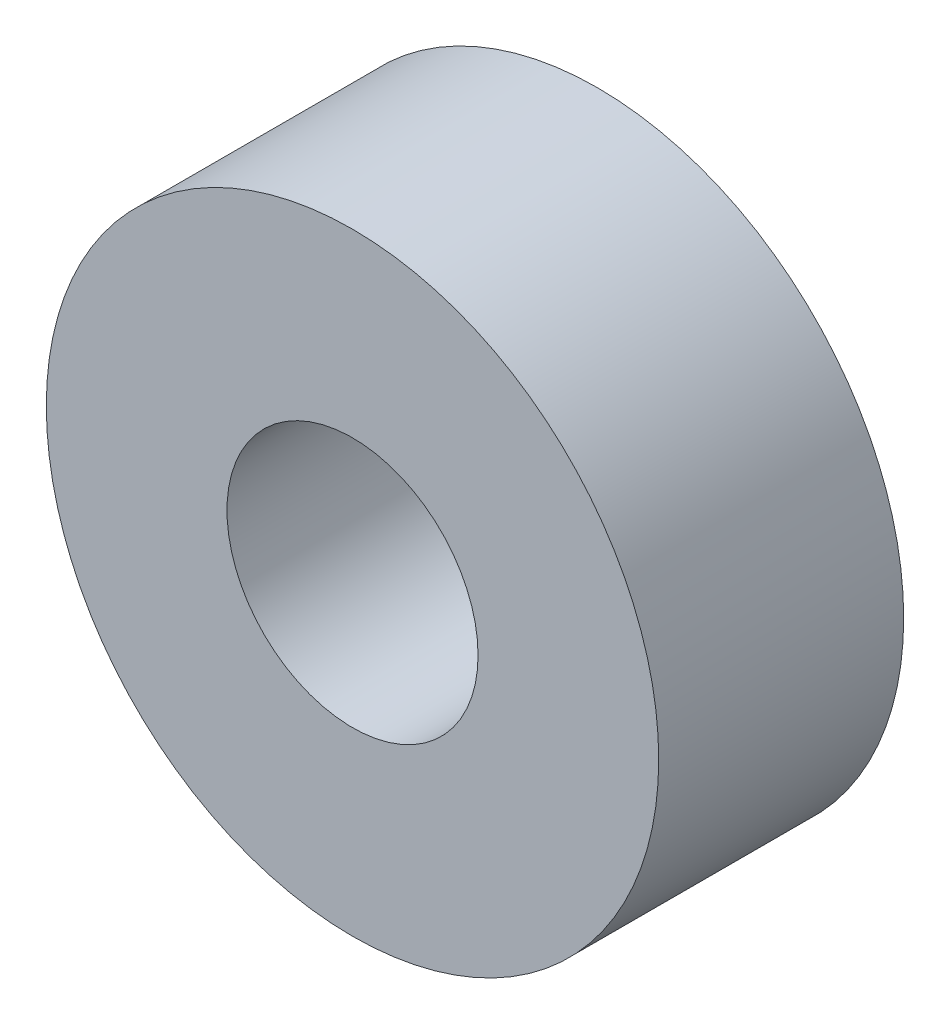
SolidWorks part; units mm, degrees
ref_plane "前视基准面" through (0, 0, 0) normal (0, 0, 1) x (1, 0, 0)
ref_plane "上视基准面" through (0, 0, 0) normal (0, 1, 0) x (1, 0, 0)
ref_plane "右视基准面" through (0, 0, 0) normal (1, 0, 0) x (0, 0, -1)
other "Configuration Table"
sketch "草图1" plane through (0, 0, 0) normal (0, 0, 1) x (1, 0, 0)
  circle A0 centre (0, 0) radius 20
  circle A1 centre (0, 0) radius 8.2
  point P0 (0, 0)
  dimension "D1" = 16.4
  dimension "D2" = 40
extrude "凸台-拉伸1" add sketch "草图1" against normal mid plane 16
